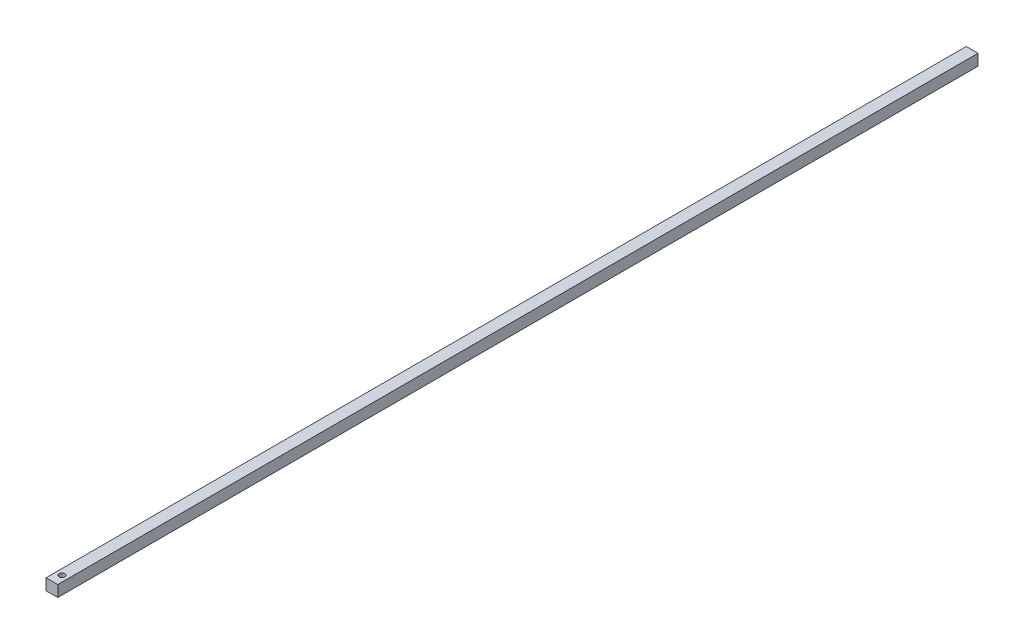
SolidWorks part; units mm, degrees
ref_plane "前视基准面" through (0, 0, 0) normal (0, 0, 1) x (1, 0, 0)
ref_plane "上视基准面" through (0, 0, 0) normal (0, 1, 0) x (1, 0, 0)
ref_plane "右视基准面" through (0, 0, 0) normal (1, 0, 0) x (0, 0, -1)
sketch "草图1" plane through (0, 0, 0) normal (0, 0, 1) x (1, 0, 0)
  line L1 (11.5, -11) -> (-11.5, -11)
  line L2 (11.5, -11) -> (11.5, 11)
  line L3 (11.5, 11) -> (-11.5, 11)
  line L4 (-11.5, -11) -> (-11.5, 11)
  line L5 (11.5, -11) -> (-11.5, 11) construction
  line L6 (11.5, 11) -> (-11.5, -11) construction
  point P0 (0, 0)
  dimension "D1" = 23
  dimension "D2" = 22
extrude "凸台-拉伸1" add sketch "草图1" along normal mid plane 1800
sketch "草图2" plane through (0, 11, 0) normal (0, 1, 0) x (1, 0, 0)
  line L0 (11.5, -900) -> (-11.5, -900) construction
  circle A0 centre (0, -880) radius 5.5
  dimension "D1" = 11
  dimension "D2" = 20
extrude "切除-拉伸1" cut sketch "草图2" against normal blind 9
sketch "草图3" plane through (0, 2, 0) normal (0, 1, 0) x (1, 0, 0)
  circle A0 centre (0, -880) radius 3.5
  dimension "D1" = 7
extrude "切除-拉伸2" cut sketch "草图3" against normal up to next
